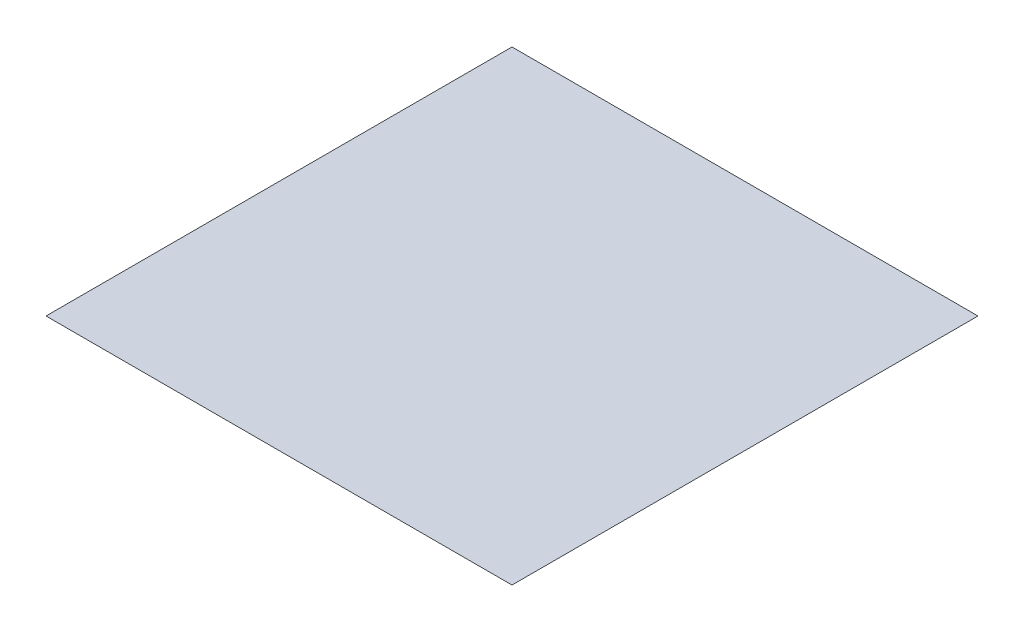
SolidWorks part; units mm, degrees
ref_plane "前视基准面" through (0, 0, 0) normal (0, 0, 1) x (1, 0, 0)
ref_plane "上视基准面" through (0, 0, 0) normal (0, 1, 0) x (1, 0, 0)
ref_plane "右视基准面" through (0, 0, 0) normal (1, 0, 0) x (0, 0, -1)
sketch "草图1" plane through (0, 0, 0) normal (0, 1, 0) x (1, 0, 0)
  line L1 (-22.75, 22.75) -> (22.75, 22.75)
  line L2 (-22.75, 22.75) -> (-22.75, -22.75)
  line L3 (-22.75, -22.75) -> (22.75, -22.75)
  line L4 (22.75, 22.75) -> (22.75, -22.75)
  line L5 (-22.75, 22.75) -> (22.75, -22.75) construction
  line L6 (-22.75, -22.75) -> (22.75, 22.75) construction
  point P0 (0, 0)
  dimension "D1" = 45.5
sketch "草图2" plane through (0, 0, 0) normal (0, 0, 1) x (1, 0, 0)
  line L0 (22.75, 0) -> (165.5648, 100)
  line L1 (-22.75, 0) -> (22.75, 0) construction
  line L2 (-22.75, 0) -> (-165.5648, 100)
  line L3 (-22.75, 0) -> (22.75, 0) construction
  line L4 (-22.75, 0) -> (22.75, 0) construction
  line L5 (-22.75, 0) -> (22.75, 0) construction
  line L6 (-165.5648, 100) -> (165.5648, 100)
  dimension "D1" = 145
  dimension "D2" = 145
  dimension "D3" = 100
sketch "草图3" plane through (0, 0, 0) normal (1, 0, 0) x (0, 0, -1)
  line L0 (-22.75, 0) -> (-165.5648, 100)
  line L1 (-22.75, 0) -> (22.75, 0) construction
  line L2 (-165.5648, 100) -> (165.5648, 100)
  line L3 (165.5648, 100) -> (22.75, 0)
  line L4 (22.75, 0) -> (-22.75, 0) construction
  dimension "D1" = 145
  dimension "D2" = 145
  dimension "D3" = 100
ref_plane "基准面4" through (0, 100, 0) normal (0, -1, 0) x (-1, 0, 0)
sketch "草图5" plane through (0, 100, 0) normal (0, -1, 0) x (-1, 0, 0)
  line L1 (165.5648, -165.5648) -> (-165.5648, -165.5648)
  line L2 (165.5648, -165.5648) -> (165.5648, 165.5648)
  line L3 (165.5648, 165.5648) -> (-165.5648, 165.5648)
  line L4 (-165.5648, -165.5648) -> (-165.5648, 165.5648)
  line L5 (165.5648, -165.5648) -> (-165.5648, 165.5648) construction
  line L6 (165.5648, 165.5648) -> (-165.5648, -165.5648) construction
  point P0 (0, 0)
loft "放样1" add profiles "草图5", "草图1"
